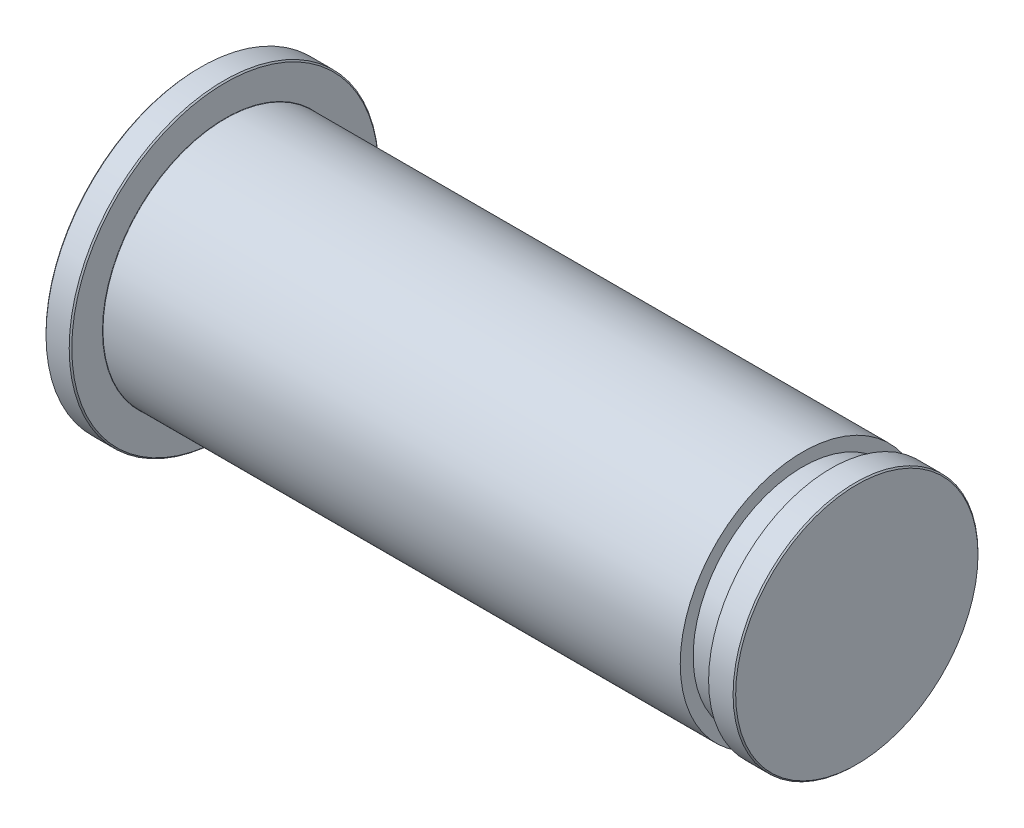
SolidWorks part; units mm, degrees
ref_plane "Front Plane" through (0, 0, 0) normal (0, 0, 1) x (1, 0, 0)
ref_plane "Top Plane" through (0, 0, 0) normal (0, 1, 0) x (1, 0, 0)
ref_plane "Right Plane" through (0, 0, 0) normal (1, 0, 0) x (0, 0, -1)
sketch "Sketch1" plane through (0, 0, 0) normal (1, 0, 0) x (0, 0, -1)
  circle A0 centre (0, 0) radius 4.75
  dimension "D1" = 9.5
extrude "Boss-Extrude1" add sketch "Sketch1" along normal blind 24.5
sketch "Sketch2" plane through (0, 0, 0) normal (-1, 0, 0) x (0, 0, 1)
  circle A0 centre (0, 0) radius 6
  dimension "D1" = 12
extrude "Boss-Extrude2" add sketch "Sketch2" along normal blind 1
chamfer "Chamfer1" distance 0.05 angle 45 2 edges at (0, 0, 6) (-1, 0, 6)
fillet "Fillet1" radius 0.01 1 edges at (0, 0, 4.75)
chamfer "Chamfer2" distance 0.05 angle 45 1 edges at (24.5, 0, -4.75)
ref_plane "Plane1" through (23.5, 0, 0) normal (1, 0, 0) x (0, 0, -1)
sketch "Sketch4" plane through (23.5, 0, 0) normal (1, 0, 0) x (0, 0, -1)
  circle A0 centre (0, 0) radius 4.25
  circle A1 centre (0, 0) radius 5.5
  dimension "D1" = 11
  dimension "D2" = 8.5
extrude "Cut-Extrude1" cut sketch "Sketch4" against normal blind 1.1
